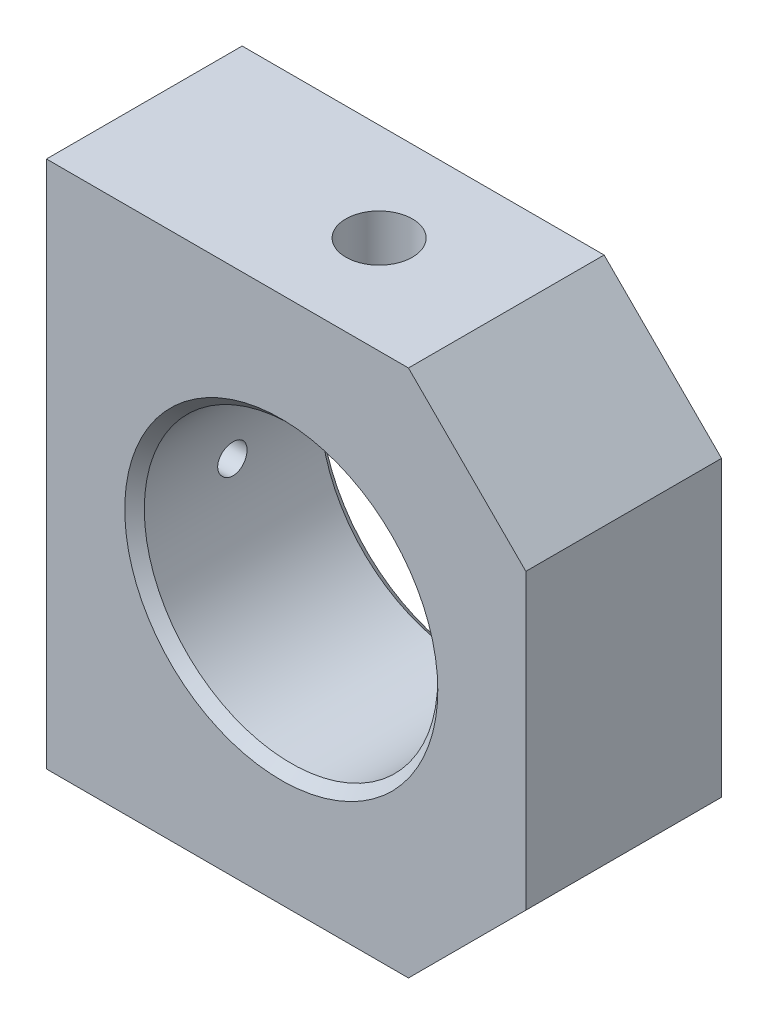
from build123d import *

# Parameters (mm, degrees)
BOSS_EXTRUDE1_DEPTH        = 20
SKETCH2_R                  = 15
CUT_EXTRUDE1_DEPTH         = 20
M8_TAPPED_HOLE1_D          = 6.8
M8_TAPPED_HOLE1_DEPTH      = 15
M8_TAPPED_HOLE1_TIP        = 2.042926105
CHAMFER2_SIZE              = 1
SIZE_MM_DOWEL_HOLE_1_D     = 3
SIZE_MM_DOWEL_HOLE_1_DEPTH = 19.75
SIZE_MM_DOWEL_HOLE_1_TIP   = 0.901290929


with BuildPart() as part:
    # Sketch1 → Boss-Extrude1 (new body)
    with BuildSketch(Plane.XY):
        Polygon((12.5, 27), (24.5, 15), (24.5, -15), (12.5, -27), (-24.5, -27), (-24.5, 27), align=None)
    extrude(amount=BOSS_EXTRUDE1_DEPTH)

    # Sketch2 → Cut-Extrude1 (cut)
    with BuildSketch(Plane.XY.offset(20)):
        with Locations((-0.5, 0)):
            Circle(SKETCH2_R)
    extrude(amount=-CUT_EXTRUDE1_DEPTH, mode=Mode.SUBTRACT)

    # M8 Tapped Hole1
    with Locations(Plane(origin=(-0.5, 27, 10), x_dir=(0, 0, 1), z_dir=(0, 1, 0))):
        with Locations((0, 0)):
            Hole(M8_TAPPED_HOLE1_D / 2, depth=M8_TAPPED_HOLE1_DEPTH)
            with Locations((0, 0, -(M8_TAPPED_HOLE1_DEPTH + M8_TAPPED_HOLE1_TIP / 2))):  # 118° drill point
                Cone(0, M8_TAPPED_HOLE1_D / 2, M8_TAPPED_HOLE1_TIP, mode=Mode.SUBTRACT)

    # Chamfer2
    chamfer2_edges = [part.edges().sort_by_distance(p)[0] for p in [
        (-15.5, 0, 0),
        (-15.5, 0, 20),
    ]]
    chamfer(chamfer2_edges, length=CHAMFER2_SIZE)

    # Size mm dowel hole 1
    with Locations(Plane(origin=(-24.5, 0, 10), x_dir=(0, -1, 0), z_dir=(-1, 0, 0))):
        with Locations((0, 0)):
            Hole(SIZE_MM_DOWEL_HOLE_1_D / 2, depth=SIZE_MM_DOWEL_HOLE_1_DEPTH)
            with Locations((0, 0, -(SIZE_MM_DOWEL_HOLE_1_DEPTH + SIZE_MM_DOWEL_HOLE_1_TIP / 2))):  # 118° drill point
                Cone(0, SIZE_MM_DOWEL_HOLE_1_D / 2, SIZE_MM_DOWEL_HOLE_1_TIP, mode=Mode.SUBTRACT)


solid = part.part
